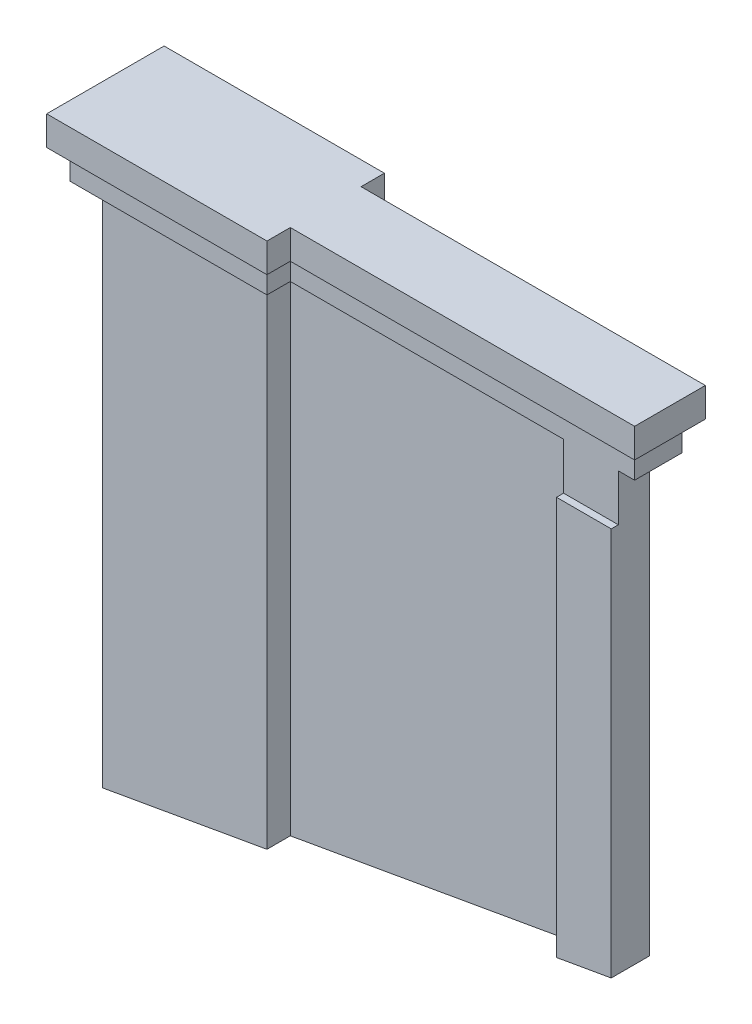
from build123d import *

# Parameters (mm, degrees)
BOSS_EXTRUDE1_DEPTH = 45
CUT_EXTRUDE1_DEPTH  = 63.941993137
BOSS_EXTRUDE2_DEPTH = 2.5
BOSS_EXTRUDE3_DEPTH = 2.5
SKETCH6_W           = 0.61
SKETCH6_H           = 4
CUT_EXTRUDE2_DEPTH  = 10


with BuildPart() as part:
    # Sketch2 → Boss-Extrude1 (new body)
    with BuildSketch(Plane(origin=(0, 0, 0), x_dir=(1, 0, 0), z_dir=(0, 1, 0))):
        Polygon((0.11, 0.11), (0.11, 5.39), (14.2, 5.39), (14.2, 3.39), (43.69, 3.39), (43.69, 0.11), (39, 0.11), (39, 2.11), (14.2, 2.11), (14.2, 0.11), align=None)
    extrude(amount=BOSS_EXTRUDE1_DEPTH)

    # Sketch3 → Cut-Extrude1 (cut, through all)
    with BuildSketch(Plane.XY.offset(-0.11)):
        Polygon((0.11, 0), (43.69, 0), (43.69, 7.684329819), align=None)
    extrude(amount=-CUT_EXTRUDE1_DEPTH, mode=Mode.SUBTRACT)

    # Sketch4 → Boss-Extrude2 (add)
    with BuildSketch(Plane(origin=(0, 45, 0), x_dir=(1, 0, 0), z_dir=(0, 1, 0))):
        Polygon((-1.28, 6.78), (-1.28, -1.28), (15.59, -1.28), (15.59, 0.72), (45.08, 0.72), (45.08, 4.78), (15.59, 4.78), (15.59, 6.78), align=None)
    extrude(amount=BOSS_EXTRUDE2_DEPTH)

    # Sketch5 → Boss-Extrude3 (add)
    with BuildSketch(Plane(origin=(0, 47.5, 0), x_dir=(1, 0, 0), z_dir=(0, 1, 0))):
        Polygon((46.08, -0.28), (46.08, 5.78), (16.59, 5.78), (16.59, 7.78), (-2.28, 7.78), (-2.28, -2.28), (16.59, -2.28), (16.59, -0.28), align=None)
    extrude(amount=BOSS_EXTRUDE3_DEPTH)

    # Sketch6 → Cut-Extrude2 (cut)
    with BuildSketch(Plane(origin=(43.69, 0, 0), x_dir=(0, 0, -1), z_dir=(1, 0, 0))):
        with Locations((0.415, 43)):
            Rectangle(SKETCH6_W, SKETCH6_H)
    extrude(amount=-CUT_EXTRUDE2_DEPTH, mode=Mode.SUBTRACT)


solid = part.part
